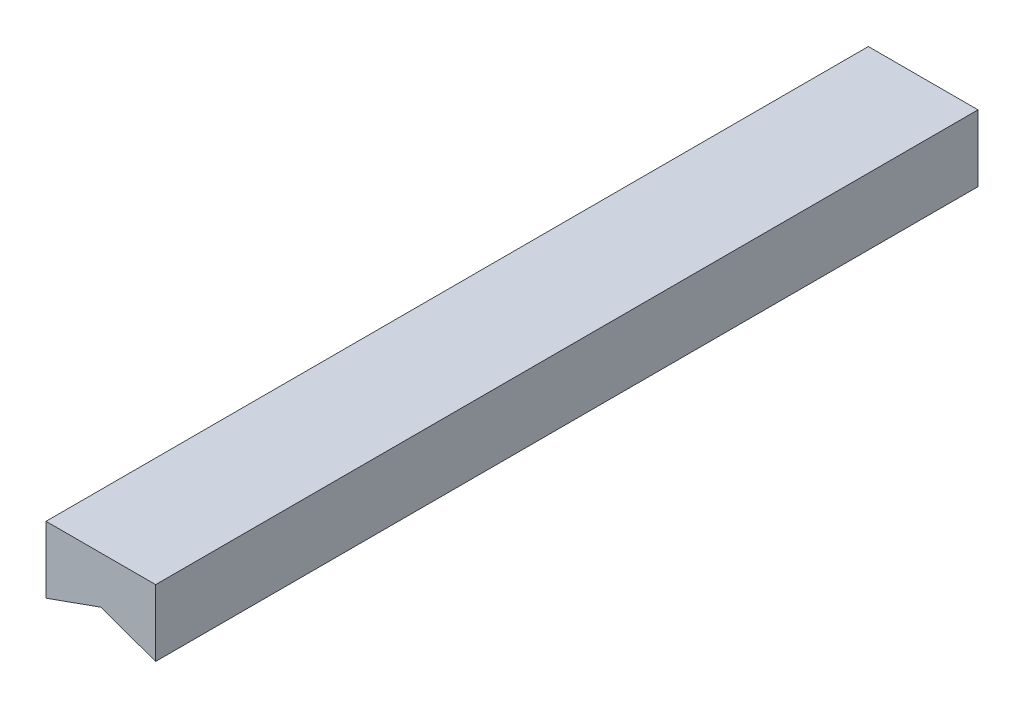
from build123d import *

# Parameters (mm, degrees)
EXTRUDE_1_DEPTH = 105


with BuildPart() as part:
    # 草图1 → 凸台-拉伸1 (new, symmetric)
    with BuildSketch(Plane.XY):
        Polygon((0, 0), (-14, -5), (-14, 12), (14, 12), (14, -5), align=None)
    extrude(amount=EXTRUDE_1_DEPTH, both=True)


solid = part.part
